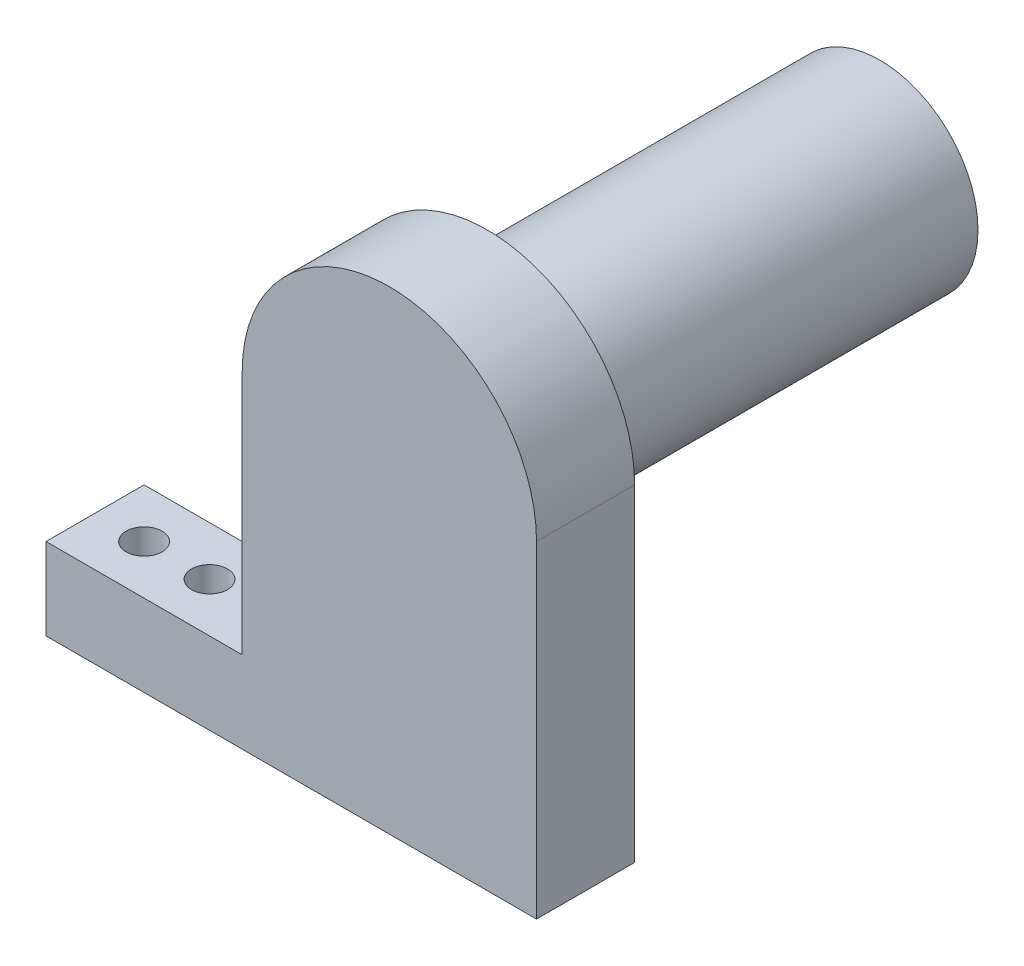
SolidWorks part; units mm, degrees
ref_plane "Front Plane" through (0, 0, 0) normal (0, 0, 1) x (1, 0, 0)
ref_plane "Top Plane" through (0, 0, 0) normal (0, 1, 0) x (1, 0, 0)
ref_plane "Right Plane" through (0, 0, 0) normal (1, 0, 0) x (0, 0, -1)
sketch "Sketch2" plane through (0, 0, 0) normal (0, 0, 1) x (1, 0, 0)
  line L1 (-75, 12.5) -> (75, 12.5)
  line L2 (-75, 12.5) -> (-75, -12.5)
  line L3 (-75, -12.5) -> (75, -12.5)
  line L4 (75, 12.5) -> (75, -12.5)
  line L5 (-75, 12.5) -> (75, -12.5) construction
  line L6 (-75, -12.5) -> (75, 12.5) construction
  point P0 (0, 0)
  dimension "D1" = 150
  dimension "D2" = 25
extrude "Boss-Extrude1" add sketch "Sketch2" along normal mid plane 30
sketch "Sketch3" plane through (0, 0, 15) normal (0, 0, 1) x (1, 0, 0)
  line L0 (75, -12.5) -> (75, 12.5) construction
  line L1 (-75, -12.5) -> (75, -12.5) construction
  line L2 (-15, 87.5) -> (-15, 0)
  line L3 (-15, 0) -> (75, 0)
  line L4 (75, 0) -> (75, 87.5)
  circle A0 centre (30, 87.5) radius 30
  arc A1 (75, 87.5) -> (-15, 87.5) centre (30, 87.5) ccw
  dimension "D1" = 60
  dimension "D2" = 90
  dimension "D3" = 100
extrude "Boss-Extrude2" add sketch "Sketch3" against normal up to surface (30 mm away) up to face at (0, 0, -15)
sketch "Sketch4" plane through (0, 12.5, 0) normal (0, 1, 0) x (1, 0, 0)
  line L0 (-75, -15) -> (-75, 15) construction
  circle A0 centre (-60, 0) radius 5.5
  circle A1 centre (-40, 0) radius 5.5
  dimension "D3" = 11
  dimension "D1" = 20
  dimension "D2" = 15
extrude "Cut-Extrude1" cut sketch "Sketch4" against normal blind 30
sketch "Sketch5" plane through (0, 0, -15) normal (0, 0, -1) x (-1, 0, 0)
  circle A0 centre (-30, 87.5) radius 30 construction
  circle A1 centre (-30, 87.5) radius 30
extrude "Boss-Extrude3" add sketch "Sketch5" along normal blind 150 from offset 30
